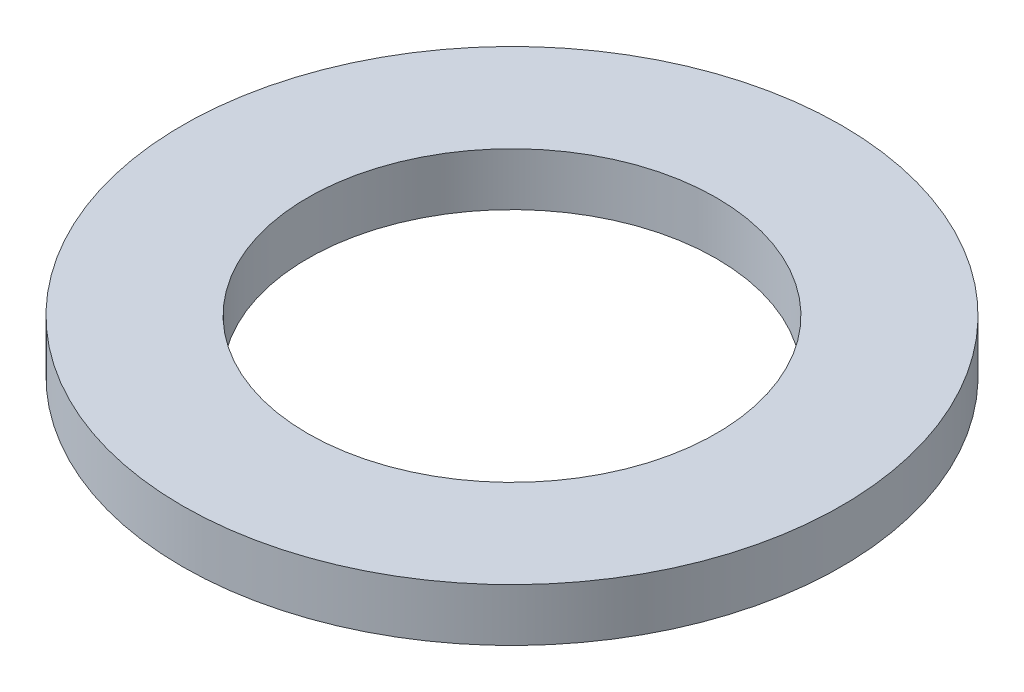
SolidWorks part; units mm, degrees
material "A3"
ref_plane "前视基准面" through (0, 0, 0) normal (0, 0, 1) x (1, 0, 0)
ref_plane "上视基准面" through (0, 0, 0) normal (0, 1, 0) x (1, 0, 0)
ref_plane "右视基准面" through (0, 0, 0) normal (1, 0, 0) x (0, 0, -1)
sketch "草图1" plane through (0, 0, 0) normal (0, 1, 0) x (1, 0, 0)
  circle A0 centre (0, 0) radius 15.5
  circle A1 centre (0, 0) radius 25
  dimension "D1" = 31
  dimension "D2" = 50
extrude "凸台-拉伸1" add sketch "草图1" along normal mid plane 4
